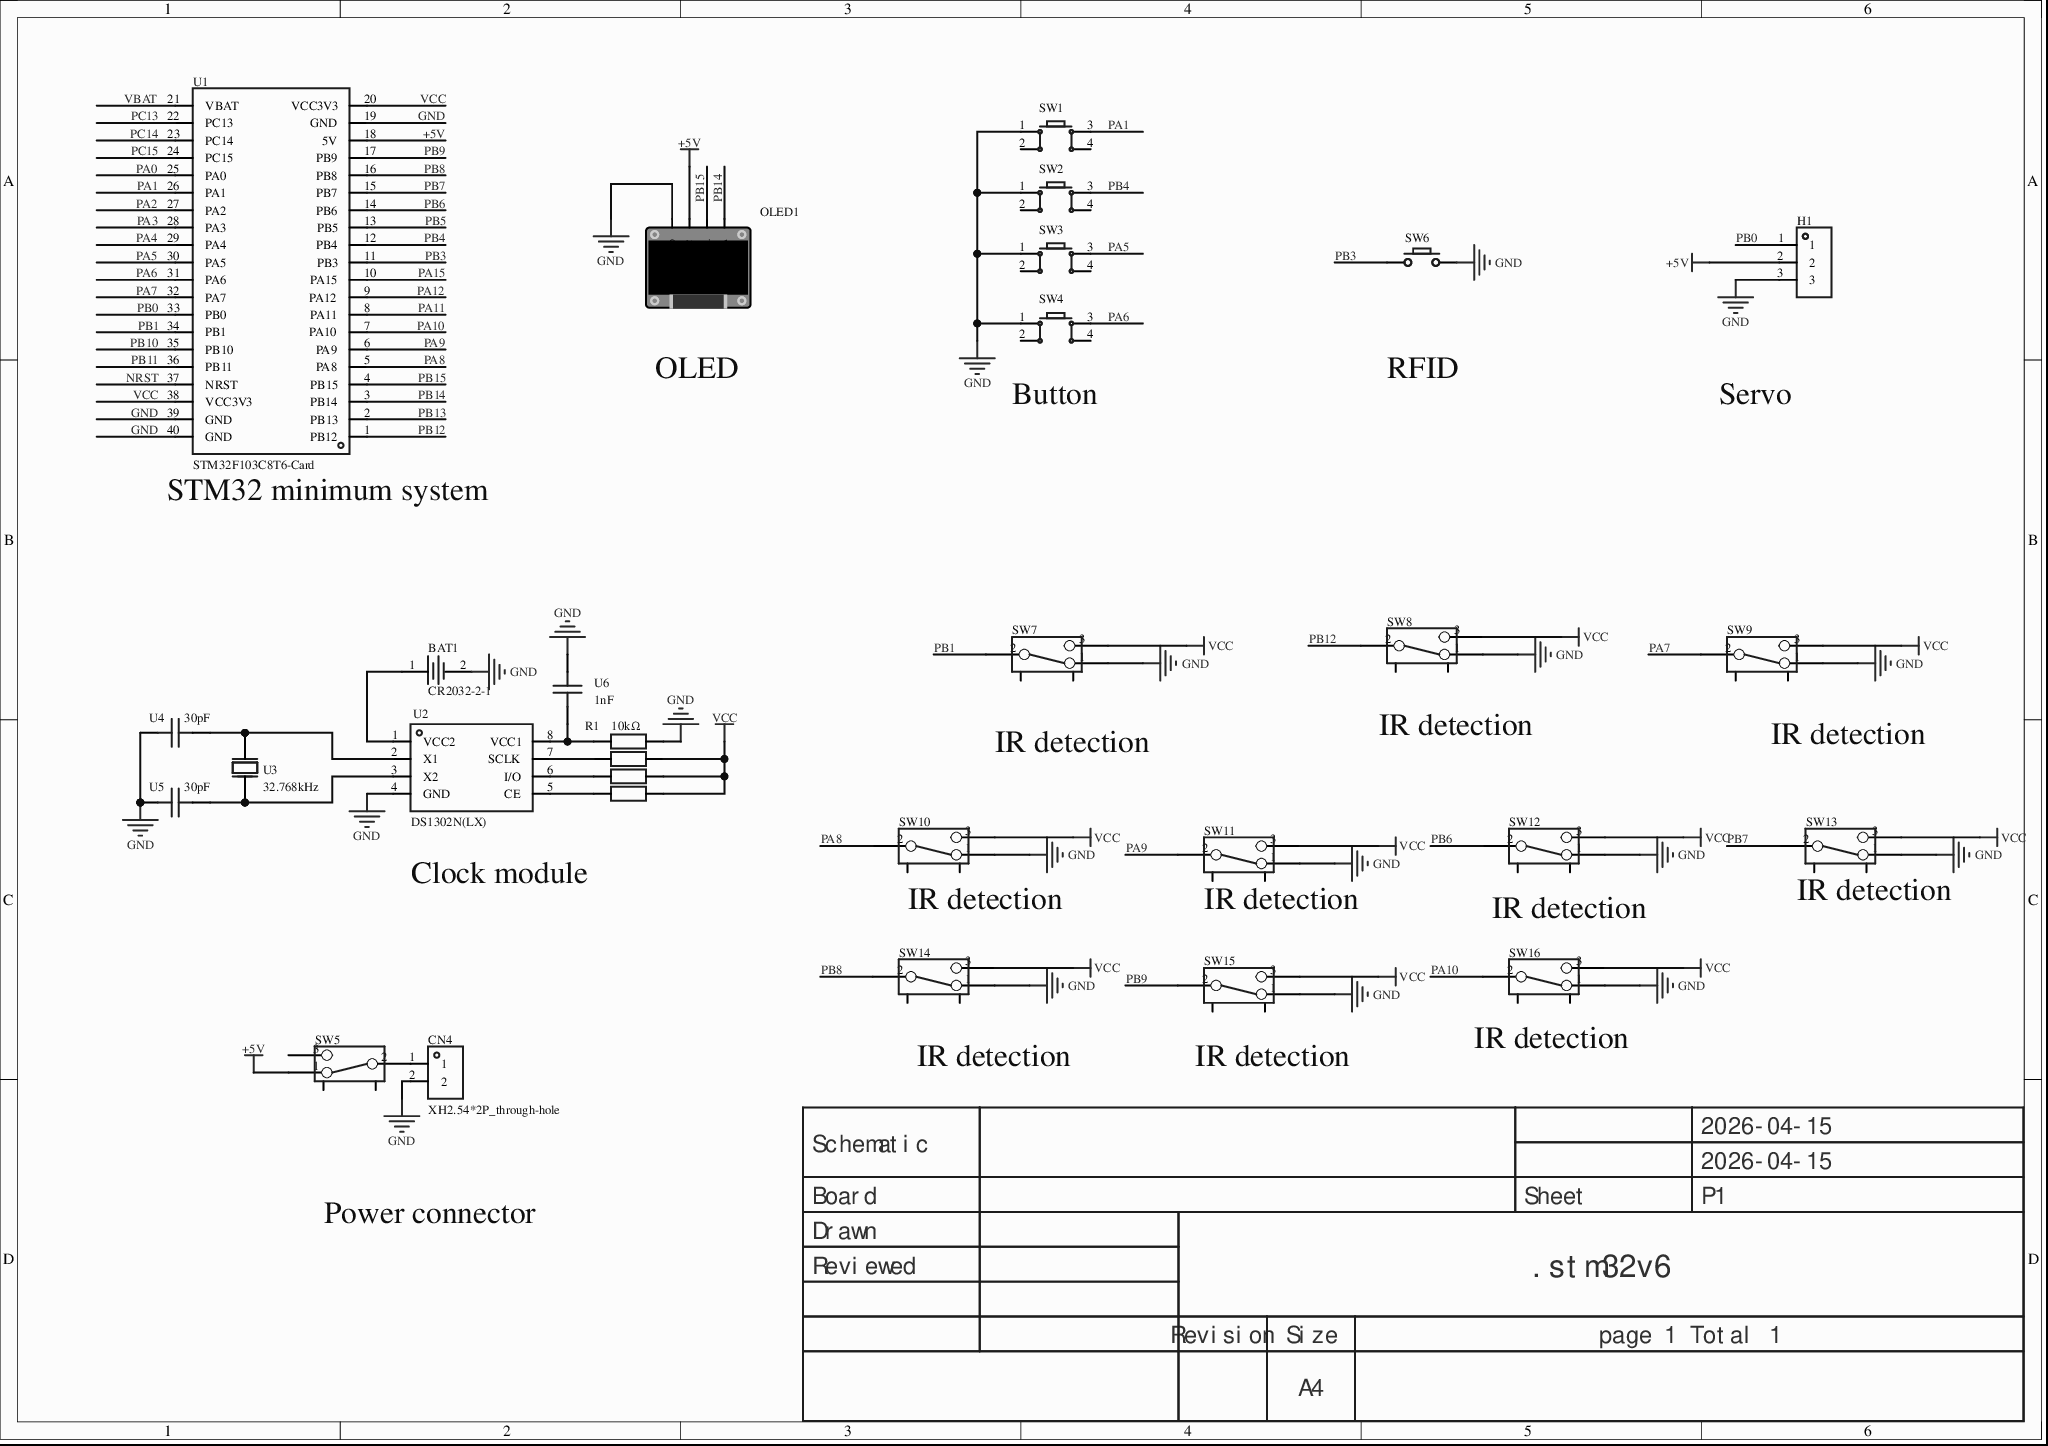
[diagram p0: MISC51813-3.schdoc]
# Altium project MISC51813-2.PrjPcb
1 sheet, 30 parts. Net scope: global (net labels, ports and power ports of the same name join across sheets).
Board file: MISC51813.pcbdoc

## Sheet MISC51813-3.schdoc
size 297 x 209 mm; Version: V1.0; @Project Name: MISC51813; @Page Count: 1; @Update Date: 2026-04-15; @Create Date: 2026-04-15; @Schematic Name: MISC51813; @Page No: 1; @Create Time: 23:22:16; @Update Time: 17:32:40; @Board Name: MISC51813

### Parts
BAT1  CR2032-2-1  [BAT-TH_CR2032-2-1]
CN4  XH2.54*2P_through-hole  [CONN-TH_2P-P2.50-XH2.54-2P]
H1  (no value)  [HDR-TH_3P-P2.54-V-F]
OLED1  (no value)  [0.96OLED_4P]
R1  10kΩ  [Res_1/8W]
R2  10kΩ  [Res_1/8W]  (value not drawn)
R3  10kΩ  [Res_1/8W]  (value not drawn)
R4  10kΩ  [Res_1/8W]  (value not drawn)
SW1  (no value)  [SW-TH_4P-L6.0-W6.0-P4.50-LS6.5]
SW2  (no value)  [SW-TH_4P-L6.0-W6.0-P4.50-LS6.5]
SW3  (no value)  [SW-TH_4P-L6.0-W6.0-P4.50-LS6.5]
SW4  (no value)  [SW-TH_4P-L6.0-W6.0-P4.50-LS6.5]
SW5  (no value)  [拨动开关]
SW6  (no value)  [Key_TH_3.5x6x4.3]
SW7  (no value)  [拨动开关]
SW8  (no value)  [拨动开关]
SW9  (no value)  [拨动开关]
SW10  (no value)  [拨动开关]
SW11  (no value)  [拨动开关]
SW12  (no value)  [拨动开关]
SW13  (no value)  [拨动开关]
SW14  (no value)  [拨动开关]
SW15  (no value)  [拨动开关]
SW16  (no value)  [拨动开关]
U1  STM32F103C8T6-Card  [CONN-TH_L53.3-W22.9_STM32F103C8T6-CARD]
U2  DS1302N(LX)  [PDIP-8_L9.3-W6.4-P2.54-LS7.9-BL-1]
U3  32.768kHz  [CRYSTAL-TH_BD2.1-P0.70-D0.3]
U4  30pF  [CAP-TH_L5.0-W2.5-P5.00-D1.0]
U5  30pF  [CAP-TH_L5.0-W2.5-P5.00-D1.0]
U6  1nF  [CAP-TH_L5.0-W2.5-P5.00-D1.0]

### Nets
+5V: H1.2 OLED1.2(VCC) SW5.1 U1.18(5V)
GND: BAT1.2 CN4.2 H1.3 OLED1.1(GND) R1.2 SW1.1 SW2.1 SW3.1 SW4.1 SW6.B SW7.1 SW8.1 SW9.1 SW10.1 SW11.1 SW12.1 SW13.1 SW14.1 SW15.1 SW16.1 U1.19(GND) U1.39(GND) U1.40(GND) U2.4(GND) U4.2 U5.2 U6.1
VCC: R2.2 R3.2 R4.2 SW7.3 SW8.3 SW9.3 SW10.3 SW11.3 SW12.3 SW13.3 SW14.3 SW15.3 SW16.3 U1.20(VCC3V3) U1.38(VCC3V3)
NRST: U1.37(NRST)
PA0: U1.25(PA0)
PA1: SW1.3 U1.26(PA1)
PA2: U1.27(PA2)
PA3: U1.28(PA3)
PA4: U1.29(PA4)
PA5: SW3.3 U1.30(PA5)
PA6: SW4.3 U1.31(PA6)
PA7: SW9.2 U1.32(PA7)
PA8: SW10.2 U1.5(PA8)
PA9: SW11.2 U1.6(PA9)
PA10: SW16.2 U1.7(PA10)
PA11: U1.8(PA11)
PA12: U1.9(PA12)
PA15: U1.10(PA15)
PB0: H1.1 U1.33(PB0)
PB1: SW7.2 U1.34(PB1)
PB3: SW6.A U1.11(PB3)
PB4: SW2.3 U1.12(PB4)
PB5: U1.13(PB5)
PB6: SW12.2 U1.14(PB6)
PB7: SW13.2 U1.15(PB7)
PB8: SW14.2 U1.16(PB8)
PB9: SW15.2 U1.17(PB9)
PB10: U1.35(PB10)
PB11: U1.36(PB11)
PB12: SW8.2 U1.1(PB12)
PB13: U1.2(PB13)
PB14: OLED1.4(SDA) U1.3(PB14)
PB15: OLED1.3(SCL) U1.4(PB15)
PC13: U1.22(PC13)
PC14: U1.23(PC14)
PC15: U1.24(PC15)
VBAT: U1.21(VBAT)
NetBAT1_1: BAT1.1 U2.1(VCC2)
NetCN4_1: CN4.1 SW5.2
NetR1_1: R1.1 U2.8(VCC1) U6.2
NetR2_1: R2.1 U2.7(SCLK)
NetR3_1: R3.1 U2.6(I/O)
NetR4_1: R4.1 U2.5(CE)
NetU2_2: U2.2(X1) U3.2 U4.1
NetU2_3: U2.3(X2) U3.1 U5.1

Not connected (* = marked no-connect by the designer): SW1 2 4; SW2 2 4; SW3 2 4; SW4 2 4; SW5 3 4 5; SW7 4 5; SW8 4 5; SW9 4 5; SW10 4 5; SW11 4 5; SW12 4 5; SW13 4 5; SW14 4 5; SW15 4 5; SW16 4 5

### Notes on the sheet
- OLED
- (near SW4) Button
- RFID
- Servo
- (near U1) STM32 minimum system
- (near SW7) IR detection
- (near SW8) IR detection
- (near SW9) IR detection
- Clock module
- (near SW10) IR detection
- (near SW11) IR detection
- IR detection
- (near SW13) IR detection
- (near SW14) IR detection
- (near SW15) IR detection
- (near SW16) IR detection
- Power connector
- 2026-04-15
- Schematic
- Board
- Sheet
- P1
- Drawn
- Reviewed
- .stm32v6
- Revision
- Size
- A4
- page 1 Total 1

### Library data of the parts
BAT1 = CR2032-2-1: AddInBom: yes; ModelId: 9f297eb2328241df835384c32afd7d320819f05c4eef4c71ace90d822a990e87; ModelTransform: 964.565,870.04,0,0,0,0,-42.047,0,-137.795; Symbol: CR2032-2-1; Device: CR2032-2-1; LCSC Part Name: CR2032-2-1; SupplierPart: C9900018737; ManufacturerPart: CR2032-2-1; Supplier Footprint: BATTERY_CR2032-A; JLCPCB Part Class: Extended Part; Supplier: LCSC; ConvertToPcb: yes; FootprintName: BAT-TH_CR2032-2-1; ModelName: BAT-TH_CR2032-2-1
CN4 = XH2.54*2P_直插: 3D Model: 325c595e30db4df8abe76612dd40b0fa0819f05c4eef4c71ace90d822a990e87; 3D Model Transform: 295.275,228.346,0,180,0,0,-0.002,-20.079,-137.795; AddInBom: yes; Symbol: XH2.54*2P_through-hole; Device: XH2.54*2P_through-hole; LCSC Part Name: XH2.54*2P_直插; Supplier Part: C9900008615; Manufacturer Part: XH2.54*2P_直插; Supplier Footprint: XH2.54_2P; JLCPCB Part Class: Extended Part; Supplier: LCSC; ConvertToPcb: yes; FootprintName: CONN-TH_2P-P2.50-XH2.54-2P; ModelName: CONN-TH_2P-P2.50-XH2.54-2P
H1 = HDR-F_2.54_1x3P: Symbol: PM254V-11-03-H85; 3D Model: f3b3cc5aae9641bf9e56fc160cef875b; 3D Model Transform: 299.9994,100,0,0,0,0,0,0,-118.11; ConvertToPcb: yes; ModelName: HDR2.54-F-LI-1X3P; Device: HDR-F_2.54_1x3P; Supplier Part: C541850; Supplier Footprint: 插件; AddInBom: yes; FootprintName: HDR-TH_3P-P2.54-V-F
OLED1 = 0.96OLED模块_4P: Symbol: 0.96OLED module_4P; ConvertToPcb: yes; ModelId: 79c000fdb68d45a296c2e9bedf4f9055; ModelTransform: 1393.69792,1318.895,0,0,0,0,0,-560.079,-137.795; Device: 0.96OLED module_4P; AddInBom: yes; FootprintName: 0.96OLED_4P; Supplier Footprint: 插件; ModelName: 0.96OLED_4P
R1-R4 = Res_AXIAL-1/8W: Symbol: Resistor; ConvertToPcb: yes; ModelId: b2b5ae7ae4c642178fe0039925c86a3f0819f05c4eef4c71ace90d822a990e87; ModelName: RES-TH_BD1.8-L3.2-P7.20-D0.4; ModelTransform: 282.86,66.88,253.09,0,0,0,0,0,-191; Device: Res_AXIAL-1/8W; AddInBom: yes; Supplier Footprint: 轴向引线; Value: 10kΩ; FootprintName: Res_1/8W
SW1-SW4 = Key_TH_6x6x6: 触点电流:50mA;额定电压(DC):12V;绝缘电阻:100MΩ;电路结构:单刀单掷;安装方式:直插;按钮形状:圆形按钮;按钮/盖帽颜色:黑色;作用力:260gf@±30gf;工作温度:-25℃~+70℃;引脚样式:PC引脚;开关长度:6mm;开关宽度:6mm;开关高度:6mm;带支架:否;; Symbol: Tactile switch; AddInBom: yes; ModelId: 20eee248bc684ccd8cbdbb1d0d91ec6f0819f05c4eef4c71ace90d822a990e87; ModelName: SW-TH_4P-L6.0-W6.0-H5.0-LS6.5-P4.50; ModelTransform: 236.22,323.03,0,90,0,0,0,0,-137.795; Device: Key_TH_6x6x6; ConvertToPcb: yes; FootprintName: SW-TH_4P-L6.0-W6.0-P4.50-LS6.5; Supplier Footprint: 插件
SW5 = 拨动开关_正: Symbol: Toggle switch; Device: Toggle switch_upright; ConvertToPcb: yes; ModelId: 4321fe59a4074cbfb4989553f297c68f0819f05c4eef4c71ace90d822a990e87; ModelName: SW-TH_SS-12D02-VG4; ModelTransform: 370.09,208.7,472.35,0,0,0,0,0,-110; AddInBom: yes; Supplier Footprint: 插件; FootprintName: Toggle switch
SW6 = Key_TH_3.5x6x4.3: ConvertToPcb: yes; ModelId: c3523f9014d949d7ba5445190a3178990819f05c4eef4c71ace90d822a990e87; ModelName: SW-TH_L6.0-W3.5-H5.0-P6.5; ModelTransform: 308.49,137.8,335.08,0,0,0,0,0,-129.92; Symbol: Key_TH_3.5x6x4.3; Device: Key_TH_3.5x6x4.3; AddInBom: yes; Supplier Footprint: 插件; FootprintName: Key_TH_3.5x6x4.3
SW7-SW16 = 拨动开关_正: Symbol: Toggle switch; Device: Toggle switch_upright; 3D Model: 4321fe59a4074cbfb4989553f297c68f0819f05c4eef4c71ace90d822a990e87; 3D Model Transform: 370.09,208.7,472.35,0,0,0,0,0,-110; ConvertToPcb: yes; ModelName: SW-TH_SS-12D02-VG4; Supplier Footprint: 插件; AddInBom: yes; FootprintName: Toggle switch
U1 = STM32F103C8T6-Card: AddInBom: yes; Symbol: STM32F103C8T6-CARD; Device: STM32F103C8T6-Card; LCSC Part Name: STM32F103C8T6-Card; SupplierPart: C9900077949; ManufacturerPart: STM32F103C8T6-Card; Supplier Footprint: 插件; Supplier: LCSC; ConvertToPcb: yes; FootprintName: CONN-TH_L53.3-W22.9_STM32F103C8T6-CARD
U2 = DS1302N(LX): DS1302是一款涓流充电时钟芯片电路，包括时钟/日历寄存器和31字节的暂存寄存器。实时时钟/日历包含秒、分、时、日期、月份和年份信息。自动调整月末日期和闰年，可选择12小时制和24小时制，可以设置AM、PM。; Manufacturer: LX(灵星芯微); AddInBom: yes; ModelId: 28221afe73f64733a5f69edf09cc82000819f05c4eef4c71ace90d822a990e87; ModelTransform: 366.141,322.834,0,0,0,0,0,0,-118.11; Voltage - Supply: 2V~5.5V; Symbol: DS1302N(LX); Device: DS1302N(LX); LCSC Part Name: DS1302N(LX); SupplierPart: C26159656; ManufacturerPart: DS1302N(LX); Supplier Footprint: DIP-8; JLCPCB Part Class: Extended Part; Datasheet: https://item.szlcsc.com/datasheet/DS1302N(LX)/27898891.html; Supplier: LCSC; ConvertToPcb: yes; FootprintName: PDIP-8_L9.3-W6.4-P2.54-LS7.9-BL-1; ModelName: PDIP-8_L9.3-W6.4-P2.54-LS7.9-BL-1; Operating Temperature: -40℃~+85℃
U3 = C-002RX 32.7680KHZ: PB FREE: 频率:32.768kHz;常温频差:±20ppm;外接负载电容:-;频率稳定度(全温):-;; AddInBom: yes; ModelId: bf3d0483db0e46329f34fee1250cddf80819f05c4eef4c71ace90d822a990e87; ModelName: OSC-TH_BD2.1-H6.0-P1.0-D0.3; ModelTransform: 291.7317,75.59,0,0,0,0,-141.733,0.003,-137.795; Normal temperature Frequency Tolerance: ±20ppm; Equivalent Series Resistance (ESR): 30kΩ; Symbol: C-002RX 32.7680KHZ: PB FREE; Device: C-002RX 32.7680KHZ: PB FREE; LCSC Part Name: 32.768kHz ±20ppm; SupplierPart: C7094009; ManufacturerPart: C-002RX 32.7680KHZ: PB FREE; Supplier Footprint: DT-26; JLCPCB Part Class: Extended Part; Datasheet: https://atta.szlcsc.com/upload/public/pdf/source/20230810/1B5E05D6078E834204F11D89EE9F3D89.pdf; Supplier: LCSC; ConvertToPcb: yes; FootprintName: CRYSTAL-TH_BD2.1-P0.70-D0.3; Value: 32.768kHz; External load capacitor: -; Frequency Stability(Full temperature range): -; Operating Temperature: -10℃~+60℃
U4-U6 = 100nF: Symbol: 100NF_C9900015256; AddInBom: yes; ModelId: 08e3d7481fc7486bb1b263873f51e1e10819f05c4eef4c71ace90d822a990e87; ModelName: CAP-TH_BD5.0-W2.5-P5.08; ModelTransform: 224.652,98.425,0,0,0,0,-0.005,0,-137.795; Device: 100nF; LCSC Part Name: 100nF; SupplierPart: C9900015256; Supplier Footprint: CAP-TH_L5.0-W2.5-P5.00-D1.0; JLCPCB Part Class: Extended Part; Supplier: LCSC; ConvertToPcb: yes; FootprintName: CAP-TH_L5.0-W2.5-P5.00-D1.0
  U4 U5: Manufacturer Part: 30pF
  U6: Manufacturer Part: 1nF